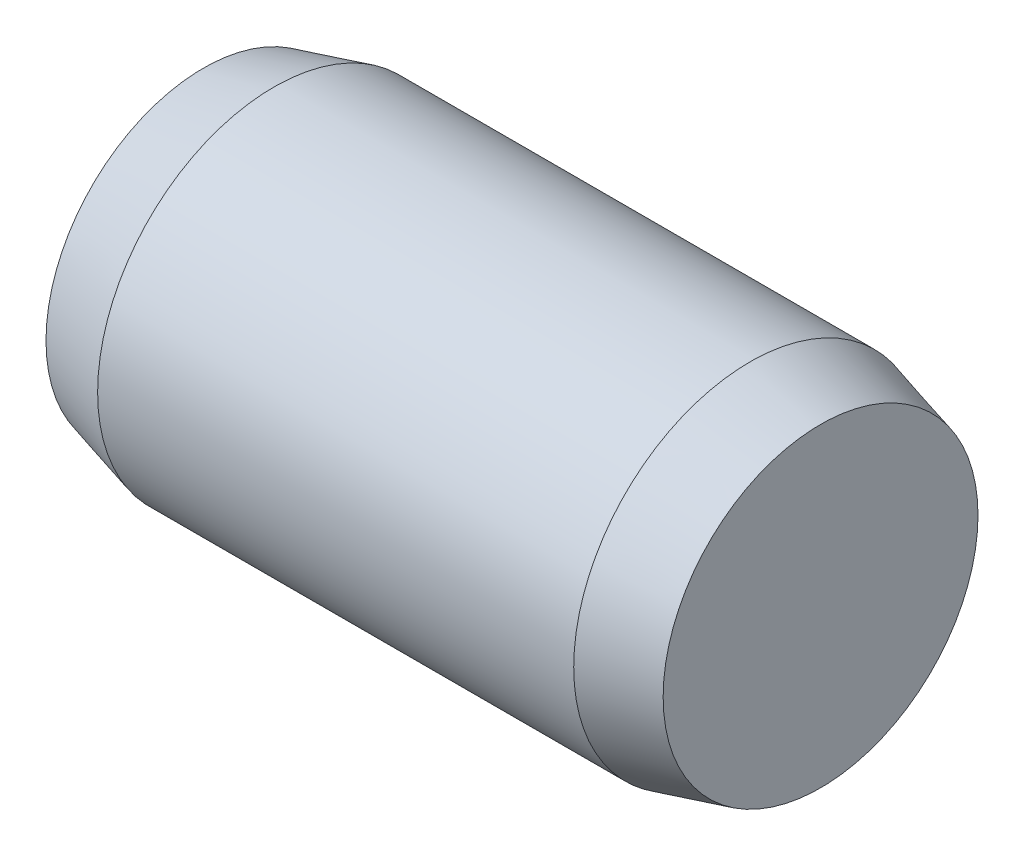
SolidWorks part; units mm, degrees
ref_plane "Front" through (0, 0, 0) normal (0, 0, 1) x (1, 0, 0)
ref_plane "Top" through (0, 0, 0) normal (0, 1, 0) x (1, 0, 0)
ref_plane "Right" through (0, 0, 0) normal (1, 0, 0) x (0, 0, -1)
sketch "Sketch1" plane through (0, 0, 0) normal (0, 0, 1) x (1, 0, 0)
  line L0 (0, 0) -> (14, 0)
  line L1 (14, 0) -> (14, 3.5713)
  line L2 (14, 3.5713) -> (12.4, 4)
  line L3 (12.4, 4) -> (1.6, 4)
  line L4 (1.6, 4) -> (0, 3.5713)
  line L5 (0, 3.5713) -> (0, 0)
  line L6 (-1.6557, 0) -> (2.6973, 0) construction
revolve "Base-Revolve" add sketch "Sketch1" angle 360 about L6
equation "\"D6@Sketch1\" = \"c@Sketch1\""
